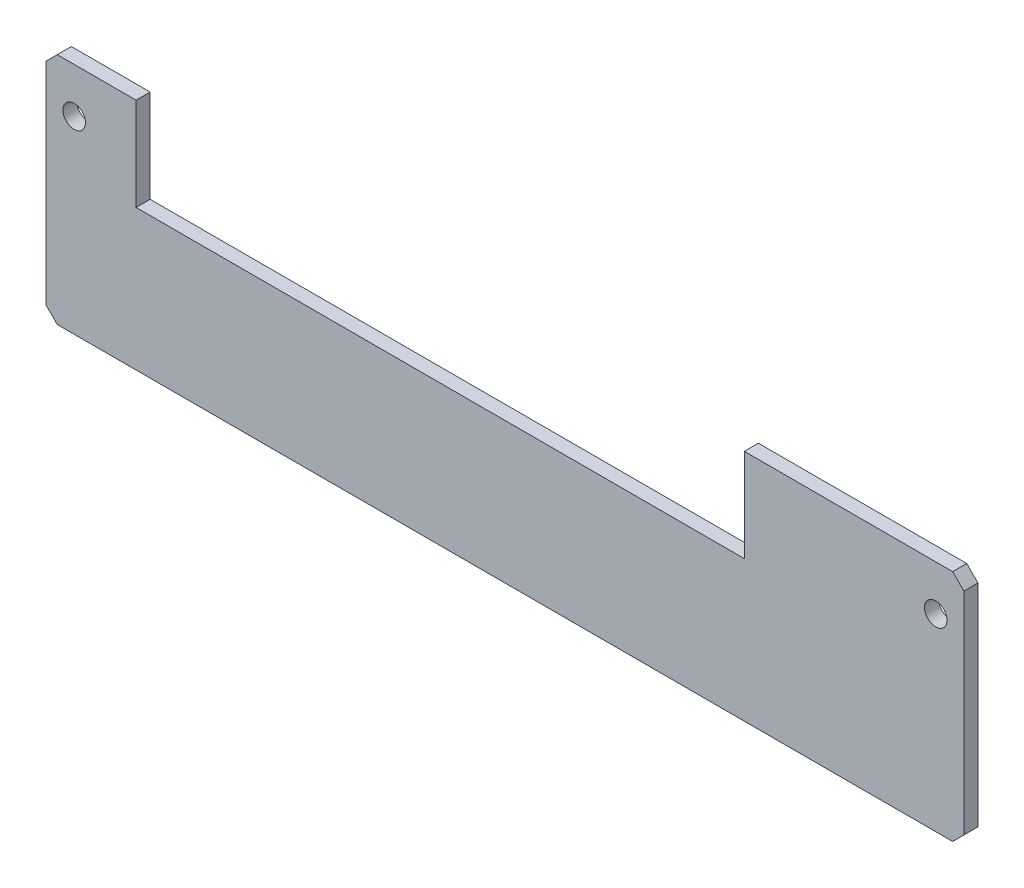
from build123d import *

# Parameters (mm, degrees)
SKETCH1_W               = 1630
SKETCH1_H               = 415
BOSS_EXTRUDE1_DEPTH     = 25
CHAMFER1_SIZE           = 20
CUT_EXTRUDE1_DEPTH      = 842.371647965
CUT_EXTRUDE1_DEPTH_BACK = 842.371647965
SKETCH2_R               = 20
SKETCH2_W               = 1080
SKETCH2_H               = 200


with BuildPart() as part:
    # Sketch1 → Boss-Extrude1 (new body)
    with BuildSketch(Plane.XY):
        Rectangle(SKETCH1_W, SKETCH1_H)
    extrude(amount=BOSS_EXTRUDE1_DEPTH)

    # Chamfer1
    chamfer1_edges = [part.edges().sort_by_distance(p)[0] for p in [
        (-815, 207.5, 12.5),
        (815, 207.5, 12.5),
        (815, -207.5, 12.5),
        (-815, -207.5, 12.5),
    ]]
    chamfer(chamfer1_edges, length=CHAMFER1_SIZE)

    # Sketch2 → Cut-Extrude1 (cut, two sides: drawn at the far end of the back side and taken through both)
    with BuildSketch(Plane.XY.offset(25).offset(-CUT_EXTRUDE1_DEPTH_BACK)):
        with Locations((-765, 127.5)):
            Circle(SKETCH2_R)
        with Locations((765, 127.5)):
            Circle(SKETCH2_R)
        with Locations((-115, 142.5)):
            Rectangle(SKETCH2_W, SKETCH2_H)
    extrude(amount=CUT_EXTRUDE1_DEPTH + CUT_EXTRUDE1_DEPTH_BACK, mode=Mode.SUBTRACT)


solid = part.part
